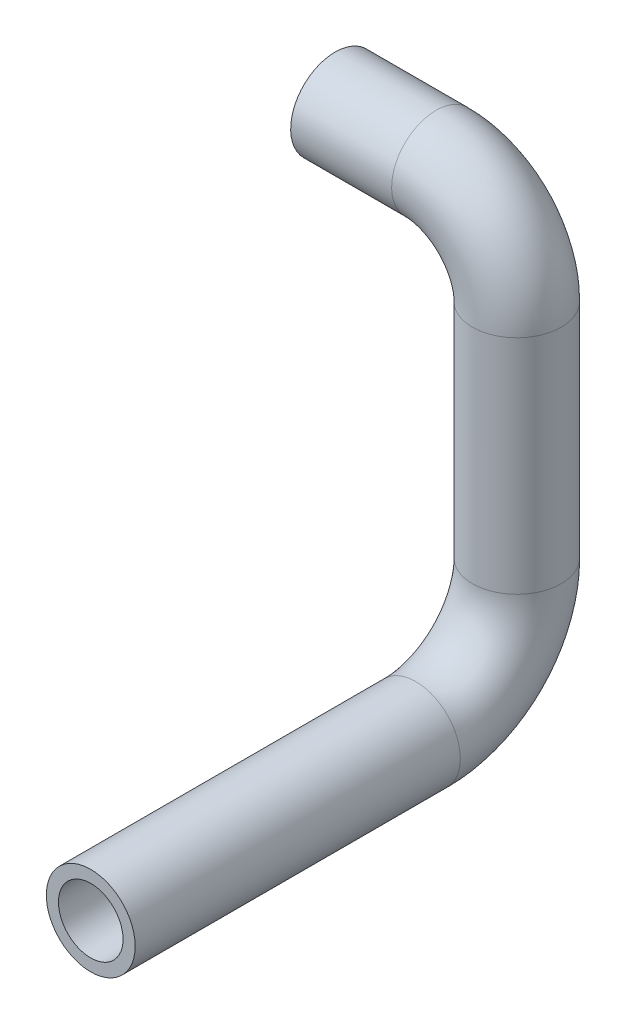
from build123d import *

# Parameters (mm, degrees)
SKETCH_2_R   = 11
SKETCH_2_R_2 = 8
SKETCH_4_R   = 11
SKETCH_4_R_2 = 8


with BuildPart() as part:
    # Sweep 1: sweep along a path in Sketch 1
    with BuildLine(Plane.XY) as sweep_1_path:
        Line((0, 0), (25, 0))
        ThreePointArc((25, 0), (39.142135624, -5.857864376), (45, -20))
        Line((45, -20), (45, -50))
    # Sketch 2 → Sweep 1 (sweep)
    with BuildSketch(Plane(origin=(0, 0, 0), x_dir=(0, 0, -1), z_dir=(1, 0, 0))):
        Circle(SKETCH_2_R)
        Circle(SKETCH_2_R_2, mode=Mode.SUBTRACT)
    sweep(path=sweep_1_path.line)

    # Sweep 2: sweep along a path in Sketch 3
    with BuildLine(Plane(origin=(45, 0, 0), x_dir=(0, 0, -1), z_dir=(1, 0, 0))) as sweep_2_path:
        Line((0, -50), (0, -75))
        ThreePointArc((0, -75), (-7.32233047, -92.67766953), (-25, -100))
        Line((-25, -100), (-105.5, -100))
    # Sketch 4 → Sweep 2 (sweep)
    with BuildSketch(Plane.XZ.offset(50)):
        with Locations((45, 0)):
            Circle(SKETCH_4_R)
        with Locations((45, 0)):
            Circle(SKETCH_4_R_2, mode=Mode.SUBTRACT)
    sweep(path=sweep_2_path.line)


solid = part.part
